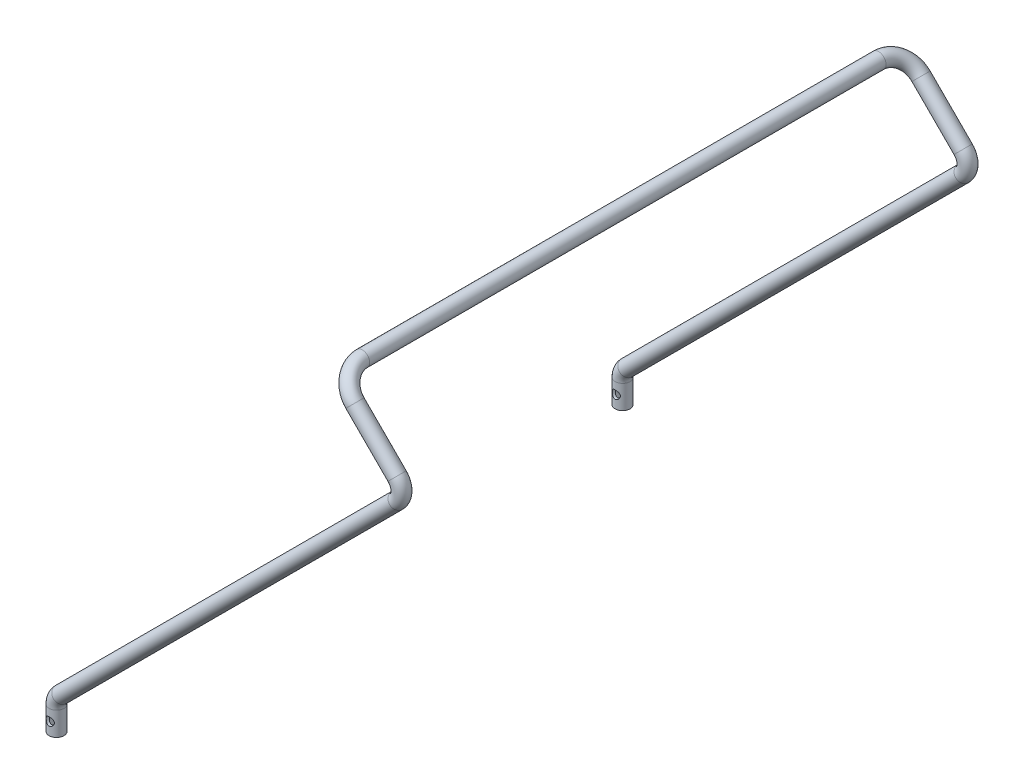
from build123d import *

# Parameters (mm, degrees)
SWEEP1_PROFILE_R        = 15
SHELL1_T                = -5
CUT_EXTRUDE1_DEPTH      = 1304.370804777
CUT_EXTRUDE1_DEPTH_BACK = 1304.370804777
SKETCH4_R               = 8.192776497


with BuildPart() as part:
    # Sweep1: sweep along a curve in space
    with BuildLine() as sweep1_path:
        Line((0, 0, 570), (0, 47.573593129, 570))
        ThreePointArc((0, 47.573593129, 570), (2.283614025, 59.0540961, 570), (8.786796564, 68.786796564, 570))
        Line((8.786796564, 68.786796564, 570), (685.893577751, 745.893577751, 570))
        ThreePointArc((685.893577751, 788.319984622, 570), (694.680374315, 767.106781187, 570), (685.893577751, 745.893577751, 570))
        Line((685.893577751, 788.319984622, 570), (601.040764009, 873.172798365, 570))
        ThreePointArc((601.040764009, 873.172798365, 570), (576.040764009, 898.172798365, 555.355339059), (565.685424949, 908.528137424, 520))
        Line((565.685424949, 908.528137424, -520), (565.685424949, 908.528137424, 520))
        ThreePointArc((565.685424949, 908.528137424, -520), (576.040764009, 898.172798365, -555.355339059), (601.040764009, 873.172798365, -570))
        Line((685.893577751, 788.319984622, -570), (601.040764009, 873.172798365, -570))
        ThreePointArc((685.893577751, 745.893577751, -570), (694.680374315, 767.106781187, -570), (685.893577751, 788.319984622, -570))
        Line((8.786796564, 68.786796564, -570), (685.893577751, 745.893577751, -570))
        ThreePointArc((8.786796564, 68.786796564, -570), (2.283614025, 59.0540961, -570), (0, 47.573593129, -570))
        Line((0, 0, -570), (0, 47.573593129, -570))
    # Sweep1 profile (on start of the path) → Sweep1 (sweep)
    with BuildSketch(Plane(origin=(0, 0, 570), x_dir=(0, 0, 1), z_dir=(0, 1, 0))):
        Circle(SWEEP1_PROFILE_R)
    sweep(path=sweep1_path.line)

    # Shell1
    shell1_openings = [part.faces().sort_by_distance(p)[0] for p in [
        (0, 0, 570),
        (0, 0, -570),
    ]]
    offset(amount=SHELL1_T, openings=shell1_openings, kind=Kind.INTERSECTION)

    # Sketch4 → Cut-Extrude1 (cut, two sides: drawn at the far end of the back side and taken through both)
    with BuildSketch(Plane.XY.offset(-CUT_EXTRUDE1_DEPTH_BACK)):
        with Locations((0, 25)):
            Circle(SKETCH4_R)
    extrude(amount=CUT_EXTRUDE1_DEPTH + CUT_EXTRUDE1_DEPTH_BACK, mode=Mode.SUBTRACT)


solid = part.part
